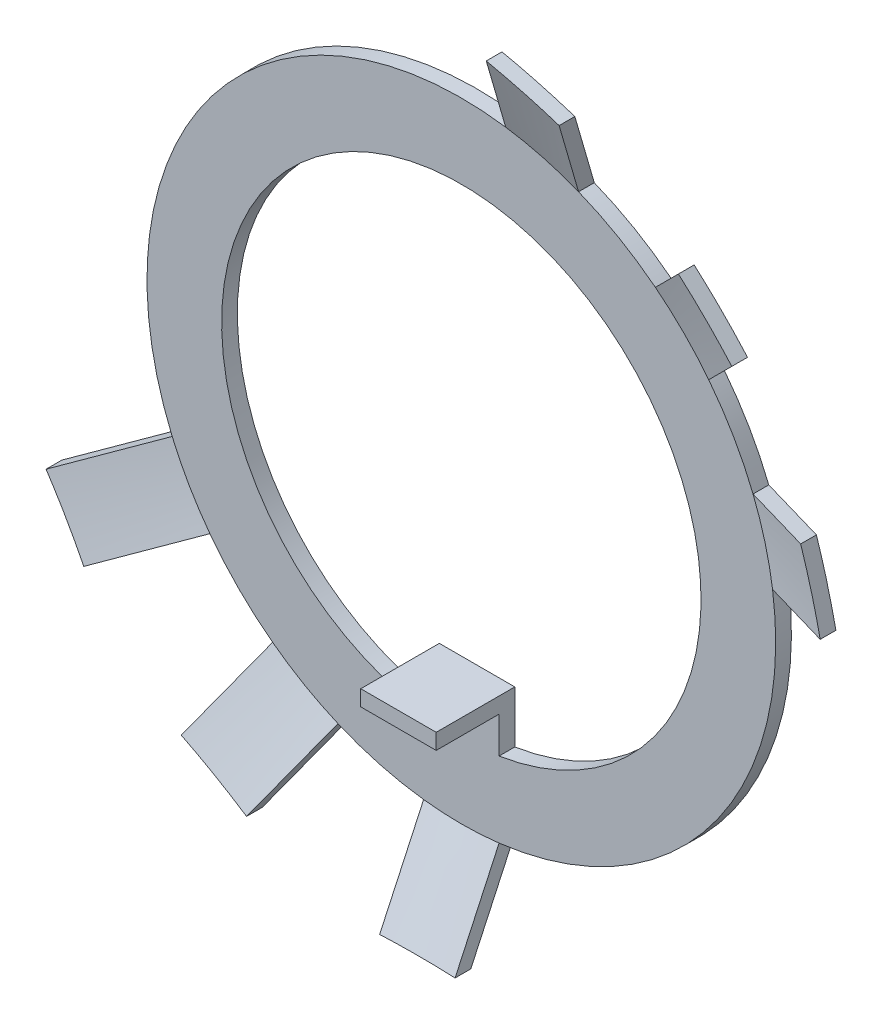
from build123d import *

# Parameters (mm, degrees)
SKETCH3_OUTSIDE_W   = 68.728
SKETCH3_OUTSIDE_H   = 68.728
CUT_EXTRUDE2_DEPTH  = 3.797865
SKETCH4_W           = 4.8
SKETCH4_H           = 1
BOSS_EXTRUDE1_DEPTH = 5


with BuildPart() as part:
    # Sketch2 → Base-Revolve (revolve)
    with BuildSketch(Plane(origin=(0, 0, 0), x_dir=(0, 0, -1), z_dir=(1, 0, 0))):
        Polygon((-2.797845949, 26), (0, 20), (0, 0), (-1, 0), (-1, 20), (-3.797845949, 26), align=None)
    revolve(axis=Axis((0, 0, 0), (0, 0, 1)))

    # Sketch3 outside → Cut-Extrude2 (cut)
    # profile 1 of 2: a face of its own
    with BuildSketch(Plane.XY):
        Rectangle(SKETCH3_OUTSIDE_W, SKETCH3_OUTSIDE_H)
        with BuildLine():
            Line((-2.4, -19.855477834), (-2.4, -25.8889938))
            Line((-2.4, -25.8889938), (2.4, -25.8889938))
            Line((2.4, -25.8889938), (2.4, -19.855477834))
            ThreePointArc((2.4, -19.855477834), (15.867066806, -12.17522858), (19.800084541, 2.82075383))
            Line((19.800084541, 2.82075383), (25.628013437, 4.382342671))
            Line((25.628013437, 4.382342671), (24.38568202, 9.018786637))
            Line((24.38568202, 9.018786637), (18.557753125, 7.457197796))
            ThreePointArc((18.557753125, 7.457197796), (17.320508076, 10), (15.736999295, 12.342886745))
            Line((15.736999295, 12.342886745), (20.003339349, 16.6092268))
            Line((20.003339349, 16.6092268), (16.6092268, 20.003339349))
            Line((16.6092268, 20.003339349), (12.342886745, 15.736999295))
            ThreePointArc((12.342886745, 15.736999295), (10, 17.320508076), (7.457197796, 18.557753125))
            Line((7.457197796, 18.557753125), (9.018786637, 24.38568202))
            Line((9.018786637, 24.38568202), (4.382342671, 25.628013437))
            Line((4.382342671, 25.628013437), (2.82075383, 19.800084541))
            ThreePointArc((2.82075383, 19.800084541), (-15.867066806, 12.17522858), (-18.395348208, -7.849277948))
            Line((-18.395348208, -7.849277948), (-23.62052631, -10.866035931))
            Line((-23.62052631, -10.866035931), (-21.22052631, -15.022957869))
            Line((-21.22052631, -15.022957869), (-15.995348208, -12.006199886))
            ThreePointArc((-15.995348208, -12.006199886), (-14.142135624, -14.142135624), (-12.006199886, -15.995348208))
            Line((-12.006199886, -15.995348208), (-15.022957869, -21.22052631))
            Line((-15.022957869, -21.22052631), (-10.866035931, -23.62052631))
            Line((-10.866035931, -23.62052631), (-7.849277948, -18.395348208))
            ThreePointArc((-7.849277948, -18.395348208), (-5.176380902, -19.318516526), (-2.4, -19.855477834))
        make_face(mode=Mode.SUBTRACT)
    # profile 2 of 2: a face of its own
    with BuildSketch(Plane.XY):
        with BuildLine():
            Line((2.4, -15.059963479), (2.4, -11.75))
            Line((2.4, -11.75), (-2.4, -11.75))
            Line((-2.4, -11.75), (-2.4, -15.059963479))
            ThreePointArc((-2.4, -15.059963479), (0, 15.25), (2.4, -15.059963479))
        make_face()
    extrude(amount=CUT_EXTRUDE2_DEPTH, mode=Mode.SUBTRACT)

    # Sketch4 → Boss-Extrude1 (add)
    with BuildSketch(Plane.XY):
        with Locations((0, -12.25)):
            Rectangle(SKETCH4_W, SKETCH4_H)
    extrude(amount=BOSS_EXTRUDE1_DEPTH)


solid = part.part
